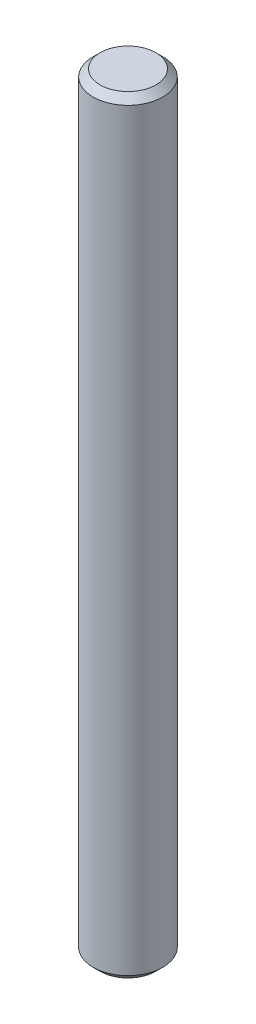
SolidWorks part; units mm, degrees
material "AISI 304"
ref_plane "前视基准面" through (0, 0, 0) normal (0, 0, 1) x (1, 0, 0)
ref_plane "上视基准面" through (0, 0, 0) normal (0, 1, 0) x (1, 0, 0)
ref_plane "右视基准面" through (0, 0, 0) normal (1, 0, 0) x (0, 0, -1)
sketch "草图1" plane through (0, 0, 0) normal (0, 1, 0) x (1, 0, 0)
  circle A0 centre (0, 0) radius 1
  dimension "D1" = 2
extrude "凸台-拉伸1" add sketch "草图1" along normal blind 22
chamfer "C0.2 倒角1" distance 0.2 angle 45 2 edges at (0, 0, 1) (0, 22, 1)
